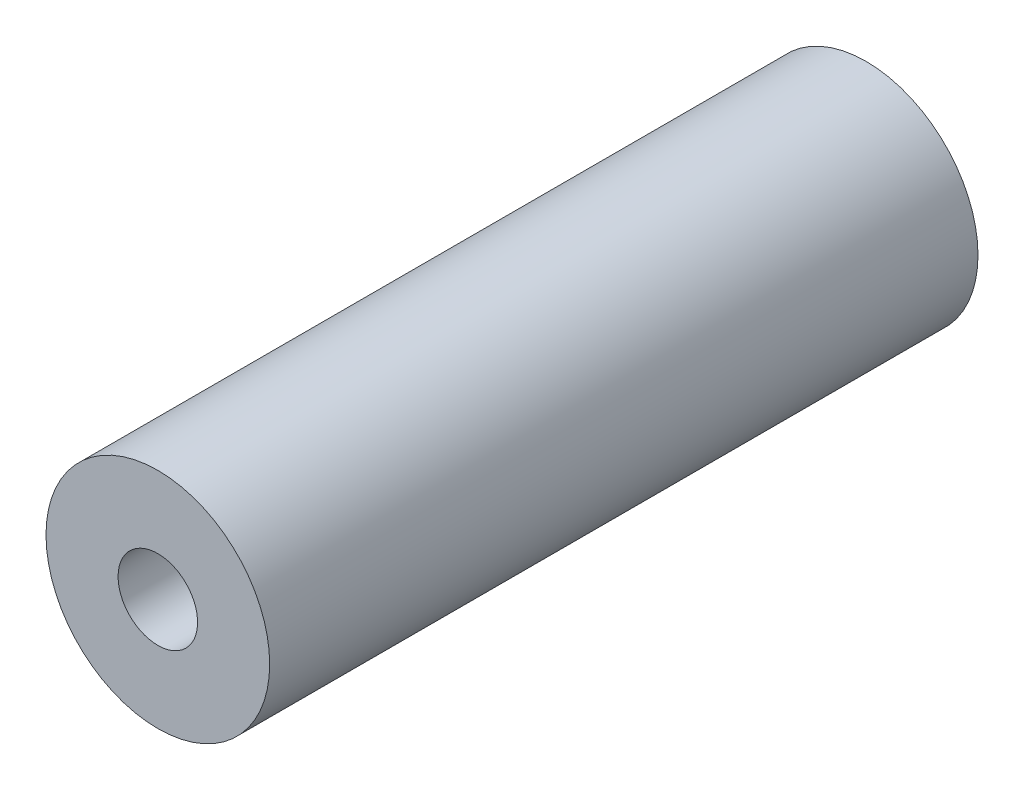
from build123d import *

# Parameters (mm, degrees)
SKETCH_1_R      = 4.5
SKETCH_1_R_2    = 1.6
EXTRUDE_1_DEPTH = 14.25


with BuildPart() as part:
    # 草图1 → 凸台-拉伸1 (new, symmetric)
    with BuildSketch(Plane.XY):
        with Locations(Location((0, 0, 0), (0, 0, 180))):
            Circle(SKETCH_1_R)
        with Locations(Location((0, 0, 0), (0, 0, 180))):
            Circle(SKETCH_1_R_2, mode=Mode.SUBTRACT)
    extrude(amount=EXTRUDE_1_DEPTH, both=True)


solid = part.part
